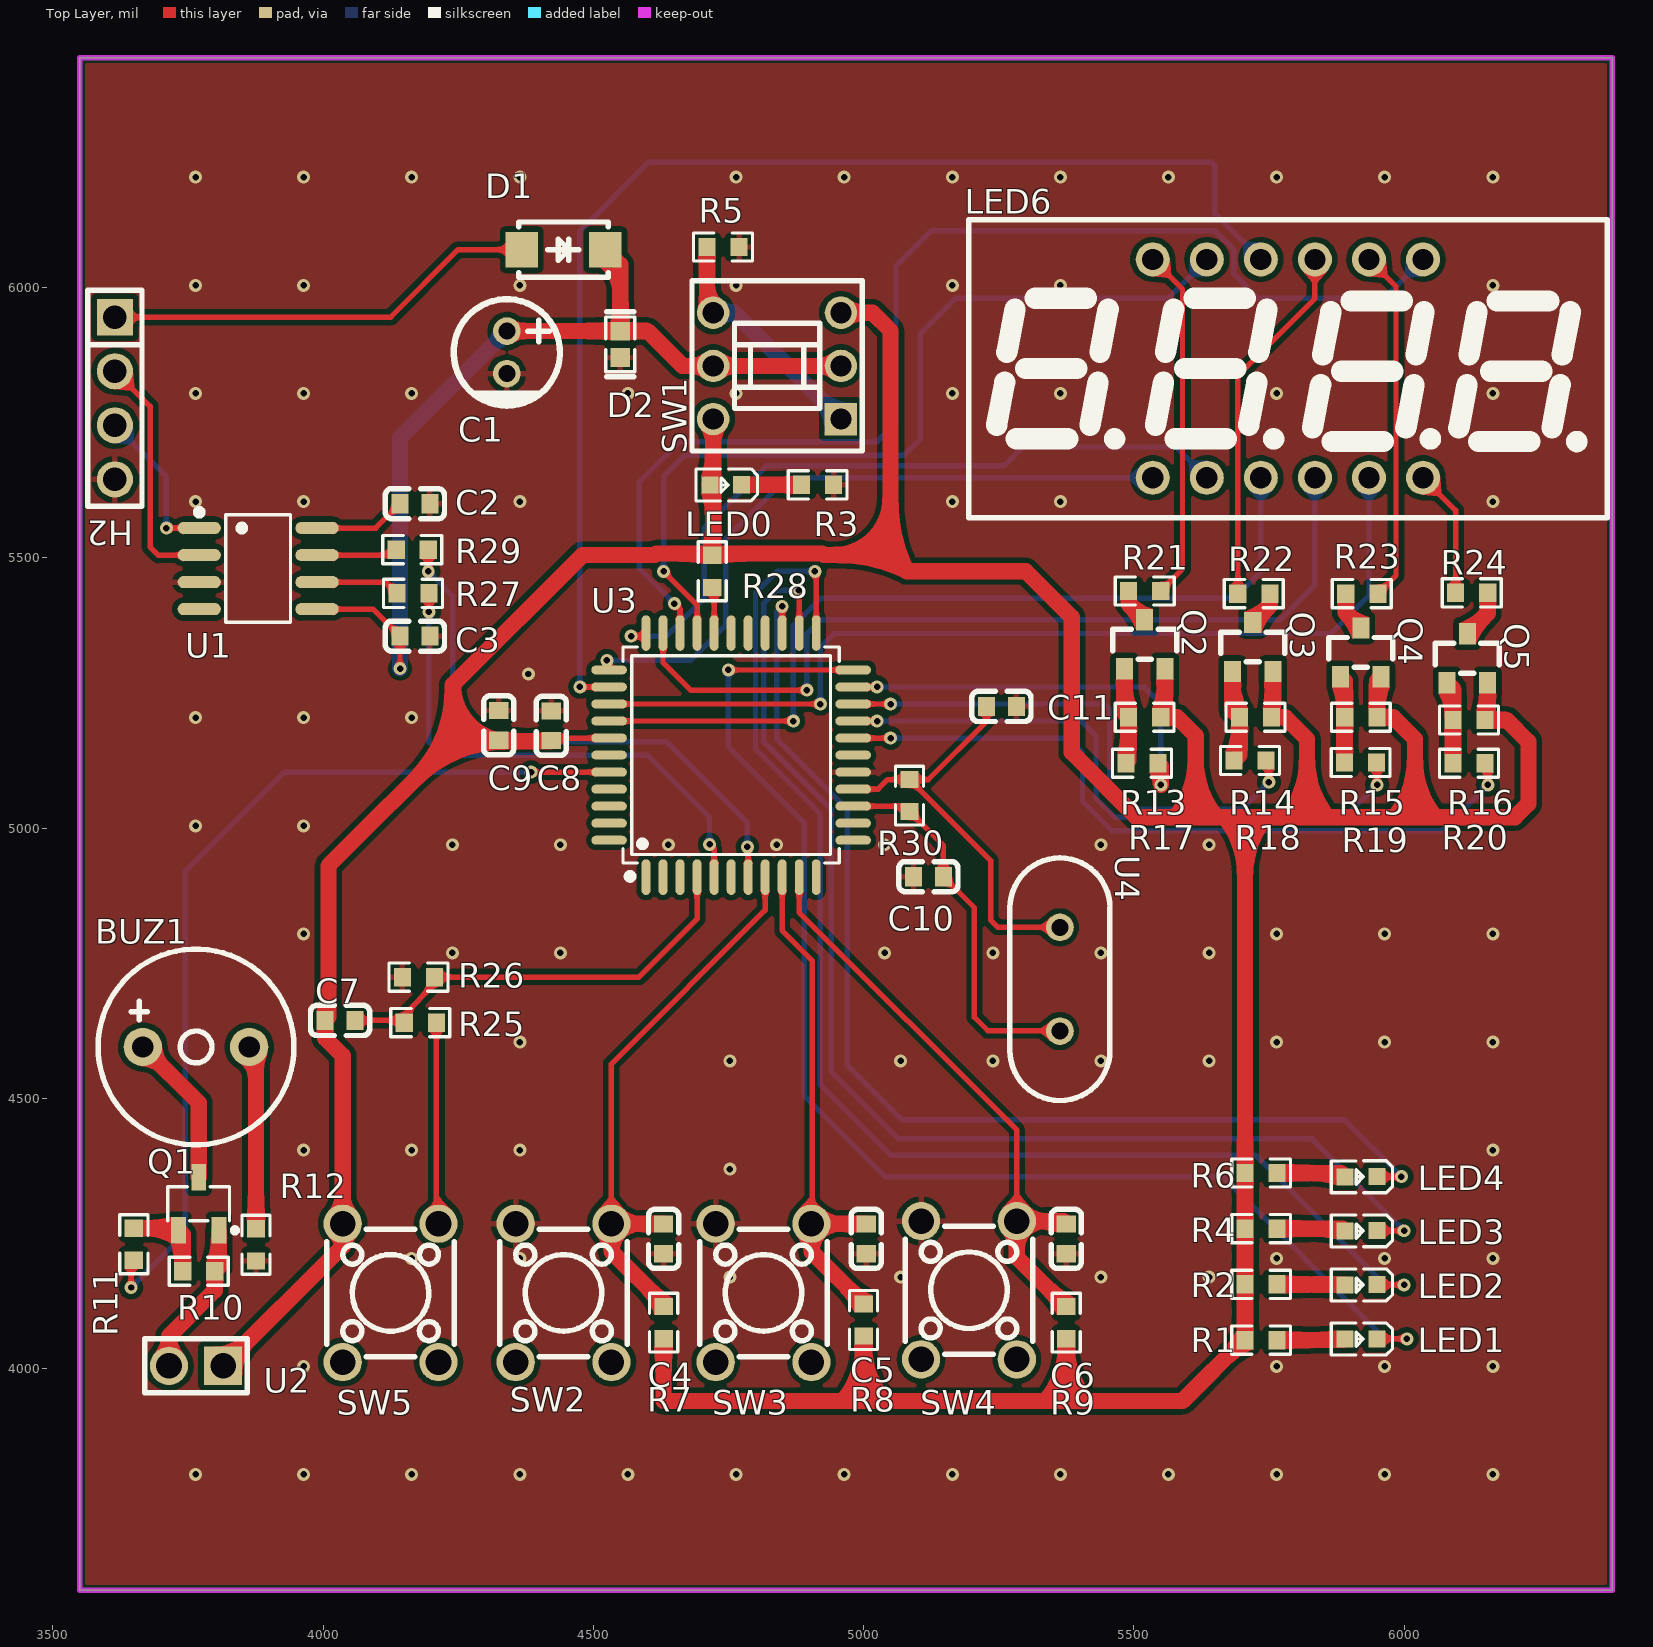
[diagram p0: Top Layer view]
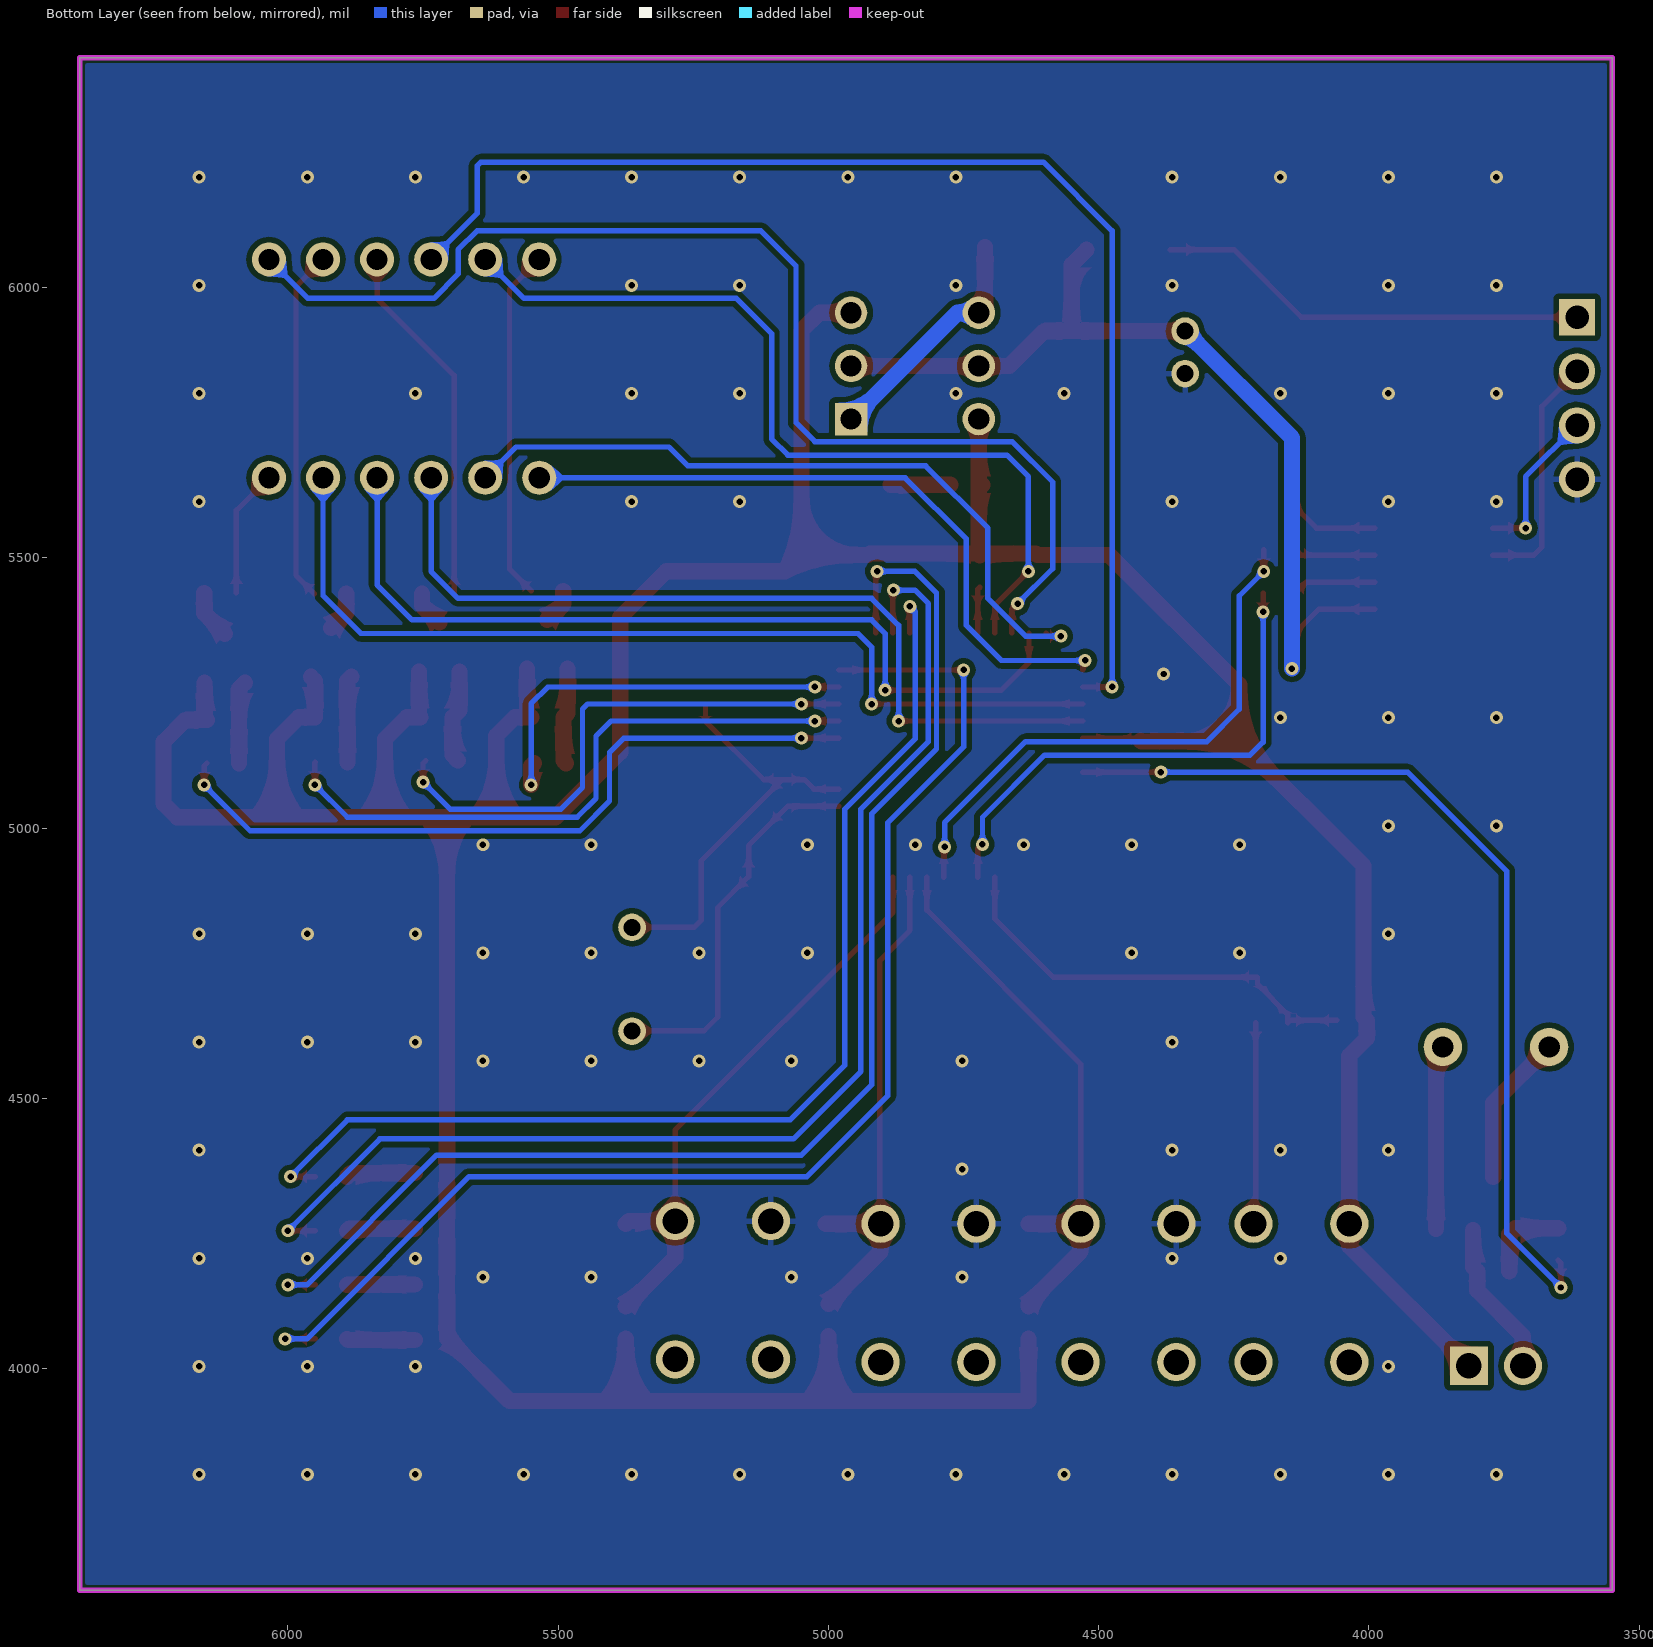
[diagram p1: Bottom Layer view, seen from below]
# Altium PCB MISC89012.pcbdoc
Units mil, origin at the board's own origin, x right, y up, seen from the top; angles counter-clockwise.
Board outline 2835 x 2835 mil, 2 copper layers (Top Layer, Bottom Layer), stack 62.206 mil thick; 65 components, 58 nets, 207 pads, 129 vias.

## Layer stack, top to bottom
Top Solder Mask Layer: solder mask 0.394, Dk 3.3
Top Layer: signal copper 1.379
Dielectric1: surface 59.449, FR4, Dk 4.5
Bottom Layer: signal copper 1.378
Bottom Solder Mask Layer: solder mask 0.394, Dk 3.3

## Board outline
3550,6425 3550,3590 6385,3590 6385,6425

## Design rules (kind name [scope] priority, off if disabled: settings)
BoardOutlineClearance copperThickness2oz_1 [All] p2 off: genericclearance=7.99 ignorepadtopadclearanceinfootprint=FALSE except(0: Arc-SplitContinuation Track-SplitContinuation SMDPad-SplitContinuation THPad-SplitContinuation Via-SplitContinuation Fill-SplitContinuation Region-SplitContinuation Poly-SplitContinuation Text-SplitContinuation Hole-SplitContinuation; 5.98: Arc-CutoutEdge SMDPad-CutoutEdge THPad-CutoutEdge Via-CutoutEdge Fill-CutoutEdge Region-CutoutEdge Text-CutoutEdge; 6.93: Hole-OutlineEdge Hole-CutoutEdge; 10: Poly-OutlineEdge Poly-CutoutEdge; 11.81: Arc-OutlineEdge Track-OutlineEdge SMDPad-OutlineEdge THPad-OutlineEdge Via-OutlineEdge Fill-OutlineEdge Region-OutlineEdge Text-OutlineEdge Track-CutoutEdge)
BoardOutlineClearance copperThickness1oz_1 [All] p4: genericclearance=4.02 ignorepadtopadclearanceinfootprint=FALSE except(0: Arc-SplitContinuation Track-SplitContinuation SMDPad-SplitContinuation THPad-SplitContinuation Via-SplitContinuation Fill-SplitContinuation Region-SplitContinuation Poly-SplitContinuation Text-SplitContinuation Hole-SplitContinuation; 6: SMDPad-CutoutEdge THPad-CutoutEdge Via-CutoutEdge Fill-CutoutEdge Region-CutoutEdge Text-CutoutEdge; 6.93: Hole-OutlineEdge Hole-CutoutEdge; 10: Poly-OutlineEdge Poly-CutoutEdge; 11.8: Arc-OutlineEdge Track-OutlineEdge SMDPad-OutlineEdge THPad-OutlineEdge Via-OutlineEdge Fill-OutlineEdge Region-OutlineEdge Text-OutlineEdge; 11.81: Arc-CutoutEdge Track-CutoutEdge)
Clearance copperThickness2oz [All] p1 off: gap=7.99 ignorepadtopadclearanceinfootprint=FALSE except(5.98: SMDPad-Track SMDPad-SMDPad THPad-Track SMDPad-THPad THPad-THPad Track-Via SMDPad-Via THPad-Via Via-Via Fill-Track Region-Track Fill-SMDPad Region-SMDPad Fill-THPad Region-THPad Fill-Via Region-Via Fill-Fill Fill-Region Region-Region Arc-Track Arc-SMDPad Arc-THPad Arc-Via Fill-Arc Region-Arc Arc-Arc Text-Track SMDPad-Text Text-THPad Text-Via Fill-Text Region-Text Arc-Text Text-Text; 6.93: Hole-Track Hole-SMDPad Hole-THPad Hole-Via Fill-Hole Region-Hole Hole-Arc Hole-Text; 10: Poly-Track Poly-SMDPad Poly-THPad Poly-Via Poly-Fill Poly-Region Poly-Poly Poly-Arc Poly-Text Poly-Hole)
Clearance copperThickness1oz [All] p3: gap=4.02 ignorepadtopadclearanceinfootprint=FALSE except(5.98: SMDPad-Track SMDPad-SMDPad THPad-Track SMDPad-THPad THPad-THPad Track-Via SMDPad-Via THPad-Via Via-Via Fill-Track Region-Track Fill-SMDPad Region-SMDPad Fill-THPad Region-THPad Fill-Via Region-Via Fill-Fill Fill-Region Region-Region; 6: Arc-Track Arc-SMDPad Arc-THPad Arc-Via Fill-Arc Region-Arc Arc-Arc Text-Track SMDPad-Text Text-THPad Text-Via Fill-Text Region-Text Arc-Text Text-Text; 6.93: Hole-Track Hole-SMDPad Hole-THPad Hole-Via Fill-Hole Region-Hole Hole-Arc Hole-Text; 10: Poly-Track Poly-SMDPad Poly-THPad Poly-Via Poly-Fill Poly-Region Poly-Poly Poly-Arc Poly-Text Poly-Hole)
Creepage creepage [All] p1: checkdistance=0 ignoreinternallayers=TRUE applytopolygonpour=TRUE
DiffPairsRouting differentialPair [All] p1: maxlimit=6 minlimit=6 mostfreqgap=6 toplayer_minwidth=5 toplayer_prefwidth=10 toplayer_maxwidth=100 toplayer_mingap=6 toplayer_prefgap=6 toplayer_maxgap=6 bottomlayer_minwidth=5 bottomlayer_prefwidth=10 bottomlayer_maxwidth=100 bottomlayer_mingap=6 bottomlayer_prefgap=6 bottomlayer_maxgap=6 maxuncoupledlength=10
HoleToHoleClearance otherClearance [All] p1: gap=11.81 allowstackedmicrovias=TRUE
Length netLength [All] p1: minlimit=0 maxlimit=0
MatchedLengths netLengthTolerance [All] p1: tolerance=1000
PasteMaskExpansion pasteMaskExpansion [All] p1: expansion=0
PlaneConnect innerPlane [All] p1: planeconnectstyle=Relief reliefexpansion=20 reliefentries=4 reliefconductorwidth=10 reliefairgap=10
PolygonConnect copperRegion [(InNet('GND'))] p1: connectstyle=Relief reliefconductorwidth=10 reliefentries=4 polygonreliefangle="90 Angle" airgapwidth=10 via.connectstyle=Relief via.reliefconductorwidth=10 via.reliefentries=4 via.polygonreliefangle="90 Angle" via.airgapwidth=10
RoutingVias viaSize [All] p1: holewidth=12.01 width=24.02 viastyle="Through Hole" minholewidth=11.81 minwidth=19.68 maxholewidth=248.03 maxwidth=393.7
SolderMaskExpansion solderMaskExpansion [IsVia] p1: expansion=-1000 istentingtop=TRUE
SolderMaskExpansion solderMaskExpansion [All] p2: expansion=2 istentingtop=FALSE
Width copperThickness2oz_2 [All] p1 off: maxlimit=100 minlimit=8 preferedwidth=10
Width copperThickness1oz_2 [All] p2: maxlimit=100 minlimit=5 preferedwidth=10

## Components (designator, comment, footprint, x,y, rotation, side; value= is the part's Value field where it differs from the comment)
BUZ1 "SUN-09055-3" BUZ-TH_BD9.0-P5.00-D0.6-FD 3765,4595 r0 top
C1 "100uF" CAP-TH_BD5.0-P2.00-D0.8-FD 4340,5880 r270 top
C2 "100nF" C0603 4170,5600 r0 top
C3 "100nF" C0603 4170,5355 r0 top
C4 "100nF" C0603 4630,4240 r90 top
C5 "100nF" C0603 5005,4240 r90 top
C6 "100nF" C0603 5375,4240 r90 top
C7 "10uF" C0603 4031.52,4644.16 r180 top
C8 "100nF" C0603 4422.16,5189.16 r270 top
C9 "10uF" C0603 4325,5190 r270 top
C10 "47pF" C0603 5120,4910 r0 top
C11 "47pF" C0603 5255,5225 r180 top
D1 "SS14" SMA_L4.2-W2.6-LS5.0-RD_1 4445,6070 r180 top
D2 "0603ESDA-05N" D0603-BI 4550,5895 r90 top
H2 "PZ254V-11-04P" HDR-TH_4P-P2.54-V-M 3615,5795 r270 top
LED0 "NCD0603R1" LED0603-RD_RED 4745,5635 r180 top
LED1 "NCD0603R1" LED0603-RD_RED 5920,4055 r180 top
LED2 "NCD0603R1" LED0603-RD_RED 5920,4155 r180 top
LED3 "NCD0603R1" LED0603-RD_RED 5920,4255 r180 top
LED4 "NCD0603R1" LED0603-RD_RED 5920,4355 r180 top
LED6 "SR410361N" LED-SEG-TH_12P-L30.0-W14.0-P2.54-S10.26-BL 5785,5850 r0 top
Q1 "2N3906S-RTK/P" SOT-23-3_L2.9-W1.6-P1.90-LS2.8-TR-CW 3770,4305 r270 top
Q2 "AO3401A" SOT-23_L2.9-W1.3-P1.90-LS2.4-BR 5520,5340 r270 top
Q3 "AO3401A" SOT-23_L2.9-W1.3-P1.90-LS2.4-BR 5720,5335 r270 top
Q4 "AO3401A" SOT-23_L2.9-W1.3-P1.90-LS2.4-BR 5920,5325 r270 top
Q5 "AO3401A" SOT-23_L2.9-W1.3-P1.90-LS2.4-BR 6116.97,5314.25 r270 top
R1 "4.7kΩ" R0603 5735.51,4052.65 r0 top
R2 "4.7kΩ" R0603 5735.51,4155.74 r0 top
R3 "4.7kΩ" R0603 4915,5635 r180 top
R4 "4.7kΩ" R0603 5735.51,4258.84 r0 top
R5 "2kΩ" R0603 4740,6075 r180 top
R6 "4.7kΩ" R0603 5735.51,4361.94 r0 top
R7 "10kΩ" R0603 4630,4085 r270 top
R8 "10kΩ" R0603 5000,4090 r270 top
R9 "10kΩ" R0603 5375,4085 r270 top
R10 "10kΩ" R0603 3770,4180 r0 top
R11 "1kΩ" R0603 3650,4230 r90 top
R12 "10Ω" R0603 3876.06,4228.97 r90 top
R13 "10kΩ" R0603 5520,5205 r0 top
R14 "10kΩ" R0603 5725,5205 r0 top
R15 "10kΩ" R0603 5920,5205 r0 top
R16 "10kΩ" R0603 6120,5200 r0 top
R17 "1kΩ" R0603 5515,5120 r180 top
R18 "1kΩ" R0603 5715,5125 r180 top
R19 "1kΩ" R0603 5919.55,5121.38 r0 top
R20 "1kΩ" R0603 6120,5120 r0 top
R21 "47Ω" R0603 5520.1,5438.62 r180 top
R22 "47Ω" R0603 5722.02,5433.62 r0 top
R23 "47Ω" R0603 5921.77,5433.62 r180 top
R24 "47Ω" R0603 6125,5435 r0 top
R25 "100Ω" R0603 4180,4640 r0 top
R26 "10kΩ" R0603 4176.52,4724.16 r0 top
R27 "1kΩ" R0603 4166.27,5434.16 r0 top
R28 "10kΩ" R0603 4720,5475 r90 top
R29 "1kΩ" R0603 4165,5515 r0 top
R30 "1MΩ" R0603 5085,5060 r270 top
SW1 "XKB8080-Z" SW-TH_6P-L8.0-W8.0-P2.50 4840,5855 r90 top
SW2 "TS-1095-A5B2-D1" SW-TH_4P-L6.0-W6.0-P4.50-LS6.5 4445,4140 r270 top
SW3 "TS-1095-A5B2-D1" SW-TH_4P-L6.0-W6.0-P4.50-LS6.5 4815,4140 r270 top
SW4 "TS-1095-A5B2-D1" SW-TH_4P-L6.0-W6.0-P4.50-LS6.5 5195,4145 r270 top
SW5 "TS-1095-A5B2-D1" SW-TH_4P-L6.0-W6.0-P4.50-LS6.5 4125,4140 r90 top
U1 "CH340N" SOP-8_L5.0-W4.0-P1.27-LS6.0-BL 3880,5480 r270 top
U2 "54102-T0600LF" HDR-TH_2P-P2.54-V-M-R2-C1-S2.54 3765,4005 r90 top
U3 "STC89C52RC-40I-LQFP44" LQFP-44_L10.0-W10.0-P0.80-LS12.0-BL 4755,5135 r0 top
U4 "12MHz" HC-49S_L11.4-W4.7-P4.88-D0.4 5363.3,4720.32 r270 top

## Footprints (in the part's own frame and the unit in brackets; to place one, negate y for a bottom-side part, rotate by r counter-clockwise, add the part's x,y. Pads: shape width x height; smd on the part's side, far side on the other; paste and mask are expansions set on the pad)
BUZ-TH_BD9.0-P5.00-D0.6-FD [mm]
  round 1.8 hole 1 copper offset 0,0: 1(-2.5,0)
  round 1.8 hole 1: 2(2.5,0)
  silkscreen extent -4.6,-4.6 4.6,4.6
C0603 [mm]
  rect 0.8x0.9 smd: 1(-0.7,0) 2(0.7,0)
  silkscreen extent -1.39,-0.71 1.39,0.71
CAP-TH_BD5.0-P2.00-D0.8-FD [mm]
  round 1.3 hole 0.8: 1(-1,0) 2(1,0)
  silkscreen extent -2.5,-2.5 2.5,2.5
D0603-BI [mil]
  rect 34.38x35.72 smd paste-3937.01 mask+2: 1(-24.47,0) 2(24.47,0)
  silkscreen extent -60,-27 60,27
HC-49S_L11.4-W4.7-P4.88-D0.4 [mm]
  round 1.3 hole 0.8 paste+0 mask+0.05: 1(-2.44,0) 2(2.44,0)
  silkscreen extent -5.7,-2.35 5.7,2.35
HDR-TH_2P-P2.54-V-M-R2-C1-S2.54 [mm]
  rect 1.8x1.8 hole 1.2: 1(0,-1.27)
  round 1.8 hole 1.2: 2(0,1.27)
  silkscreen extent -1.27,-2.41 1.27,2.41
HDR-TH_4P-P2.54-V-M [mm]
  rect 1.7x1.7 hole 1.1: 1(-3.81,0)
  round 1.7 hole 1.1: 2(-1.27,0) 3(1.27,0) 4(3.81,0)
  silkscreen extent -5.08,-1.27 5.08,1.27
LED0603-RD_RED [mm]
  rect 0.8x0.8 smd: 1(-0.749,-0.003) 2(0.749,0.003)
  silkscreen extent -1.49,-0.75 1.39,0.76
LED-SEG-TH_12P-L30.0-W14.0-P2.54-S10.26-BL [mm]
  round 1.6 hole 1: 1(-6.35,-5.13) 2(-3.81,-5.13) 3(-1.27,-5.13) 4(1.27,-5.13) 5(3.81,-5.13) 6(6.35,-5.13) 7(6.35,5.13) 8(3.81,5.13) 9(1.27,5.13) 10(-1.27,5.13) 11(-3.81,5.13) 12(-6.35,5.13)
  silkscreen extent -15,-7 15,7
LQFP-44_L10.0-W10.0-P0.80-LS12.0-BL [mm]
  oval 0.42x1.67 smd: 1(-4,-5.735) 2(-3.2,-5.735) 3(-2.4,-5.735) 4(-1.6,-5.735) 5(-0.8,-5.735) 6(0,-5.735) 7(0.8,-5.735) 8(1.6,-5.735) 9(2.4,-5.735) 10(3.2,-5.735) 11(4,-5.735) 23(4,5.735) 24(3.2,5.735) 25(2.4,5.735) 26(1.6,5.735) 27(0.8,5.735) 28(0,5.735) 29(-0.8,5.735) 30(-1.6,5.735) 31(-2.4,5.735) 32(-3.2,5.735) 33(-4,5.735)
  oval 1.67x0.42 smd: 12(5.735,-4) 13(5.735,-3.2) 14(5.735,-2.4) 15(5.735,-1.6) 16(5.735,-0.8) 17(5.735,0) 18(5.735,0.8) 19(5.735,1.6) 20(5.735,2.4) 21(5.735,3.2) 22(5.735,4) 34(-5.735,4) 35(-5.735,3.2) 36(-5.735,2.4) 37(-5.735,1.6) 38(-5.735,0.8) 39(-5.735,0) 40(-5.735,-0.8) 41(-5.735,-1.6) 42(-5.735,-2.4) 43(-5.735,-3.2) 44(-5.735,-4)
  silkscreen extent -5.08,-5.85 5.08,5.08
R0603 [mil]
  rect 31.75x34.02 smd paste-3937.01 mask+2: 1(-29.66,0) 2(29.66,0)
  silkscreen extent -55,-26 55,26
SMA_L4.2-W2.6-LS5.0-RD_1 [mm]
  rect 1.52x1.68 smd: 1(-1.965,0) 2(1.965,0)
  silkscreen extent -2.1,-1.3 2.1,1.3
SOP-8_L5.0-W4.0-P1.27-LS6.0-BL [mil]
  oval 22.6x80.14 smd: 1(-75,-108.97) 2(-25,-108.97) 3(25,-108.97) 4(75,-108.97) 5(75,108.97) 6(25,108.97) 7(-25,108.97) 8(-75,108.97)
  silkscreen extent -110,-115 99,60
SOT-23-3_L2.9-W1.6-P1.90-LS2.8-TR-CW [mm]
  rect 1.25x0.7 smd: 1(1.25,0.95) 2(1.25,-0.95) 3(-1.25,0)
  silkscreen extent -0.8,-1.45 1.37,1.82
SOT-23_L2.9-W1.3-P1.90-LS2.4-BR [mm]
  rect 1x0.8 smd: 1(1.15,-0.95) 2(1.15,0.95) 3(-1.15,0)
  silkscreen extent -0.7,-1.5 0.7,1.5
SW-TH_4P-L6.0-W6.0-P4.50-LS6.5 [mm]
  round 1.8 hole 1.2: 1(-3.25,2.25) 2(3.25,2.25) 3(-3.25,-2.25) 4(3.25,-2.25)
  silkscreen extent -3,-3 3,3
SW-TH_6P-L8.0-W8.0-P2.50 [mm]
  rect 1.524x1.524 hole 1: 1(-2.5,-3)
  round 1.524 hole 1: 2(0,-3) 3(2.5,-3) 4(-2.5,3) 5(0,3) 6(2.5,3)
  silkscreen extent -4,-4 4,4

## Via types
v1: diameter 24.02, hole 12, Top Layer to Bottom Layer, 129 vias

## Nets (pads, with @x,y where several pads share a name; then routed paths per layer and width w, separated by ;. In a path a pad name is that pad's centre, name@x,y a point inside that pad or via, vN(x,y) a via of type N, cw(c..) or ccw(c..) an arc to the next point about the centre after c; other vN are vias at no path point)
$1N1: D1.2 H2.1 | length 804.4
  Top Layer w10: H2.1 4125,5945 4250,6070 D1.2
$1N12: C2.1 U1.8 | length 172.1
  Top Layer w10: U1.8 4097.44,5555 C2.1
$1N15: LED0.1 R3.2 | length 110.9
  Top Layer w30: LED0.1 4885.2,5635.14 R3.2
$1N23: R5.2 SW1.1 SW1.6 | length 444.1
  Top Layer w30: R5.2 4710.34,5964.98 SW1.6
  Bottom Layer w30: SW1.6 4761.26,5953.43 SW1.1
$1N27: LED1.2 R1.2 | length 126.3
  Top Layer w30: R1.2 5888.29,4052.65 LED1.2
$1N28: LED2.2 R2.2 | length 125.7
  Top Layer w30: R2.2 5889.63,4155.74 LED2.2
$1N29: LED3.2 R4.2 | length 127
  Top Layer w30: R4.2 5886.54,4258.84 LED3.2
$1N30: LED4.2 R6.2 | length 128.3
  Top Layer w30: R6.2 5883.44,4361.94 LED4.2
$1N45: BUZ1.2 R12.2 | length 341.6
  Top Layer w30: BUZ1.2 3876.06,4582.36 R12.2
$1N47: BUZ1.1 Q1.3 | length 283.6
  Top Layer w30: BUZ1.1 3770,4491.57 Q1.3
$1N48: Q1.2 R10.1 R11.2 | length 163.2
  Top Layer w30: R11.2 3728.74,4259.66 Q1.2 3740.34,4248.06 R10.1
$1N50: Q1.1 R10.2 U2.2 | length 289.1
  Top Layer w30: U2.2 3715,4060 3799.66,4144.66 R10.2 3807.4,4187.74 Q1.1
$1N61: R28.1 U3.29 | length 86
  Top Layer w10: R28.1 4723.5,5441.84 U3.29
$1N75: R27.2 U3.5 | length 966.1
  Top Layer w10: v1(4195.93,5400) R27.2 ; v1(4715,4970) 4723.5,4961.5 U3.5
  Bottom Layer w10: v1(4195.93,5400) 4195.93,5159.07 4220,5135 4600,5135 4715,5020 v1(4715,4970)
$1N76: R29.2 U3.7 | length 1047.2
  Top Layer w10: v1(4194.66,5475) R29.2 ; v1(4785,4965) 4786.5,4963.5 U3.7
  Bottom Layer w10: v1(4194.66,5475) 4240,5429.66 4240,5220 4300,5160 4635,5160 4785,5010 v1(4785,4965)
$1N86: R25.2 SW5.4 | length 373.7
  Top Layer w10: R25.2 4209.66,4271.87 SW5.4
$1N99: Q2.1 R13.1 R17.2 | length 180
  Top Layer w30: Q2.1 5482.6,5212.74 R13.1 5490.34,5125 R17.2
$1N101: Q3.1 R14.1 R18.2 | length 174.1
  Top Layer w30: Q3.1 5682.6,5217.74 R14.1 5695.34,5135 R18.2
$1N104: Q5.1 R16.1 R20.1 | length 153.4
  Top Layer w30: Q5.1 6090.34,5258.21 R16.1 R20.1
$1N106: Q4.1 R15.1 R19.1 | length 161.7
  Top Layer w30: Q4.1 5890.34,5271.98 R15.1 5889.89,5204.55 R19.1
$1N115: LED6.12 R21.1 | length 652.8
  Top Layer w10: LED6.12 5590,5996.97 5590,5478.87 R21.1
$1N116: LED6.9 R22.1 | length 677.4
  Top Layer w10: R22.1 5692.36,5837.36 5835,5980 LED6.9
$1N117: LED6.8 R23.1 | length 653
  Top Layer w10: LED6.8 5985,6001.97 5985,5467.2 R23.1
$1N118: LED6.6 R24.1 | length 238
  Top Layer w10: LED6.6 6095.34,5587.69 R24.1
$1N120: C10.2 R30.2 U3.14 U4.2 | length 707.4
  Top Layer w10: U3.14 5074.83,5040.51 R30.2 5147.56,4967.78 C10.2 5205,4852.56 5205,4650 5230,4625 5362.56,4625 U4.2
$1N121: C11.2 R30.1 U3.15 U4.1 | length 781.9
  Top Layer w10: U3.15 5027.01,5072.01 5044.66,5089.66 R30.1 ; C11.2 5227.44,5197.44 5119.66,5089.66 R30.1 ; U4.1 5248.62,4816.38 5235,4830 5235,4939.66 R30.1
$1N123: Q2.3 R21.2 | length 65.6
  Top Layer w30: R21.2 5490.44,5414.84 Q2.3
$1N124: Q3.3 R22.2 | length 66.5
  Top Layer w30: Q3.3 5751.68,5411.95 R22.2
$1N125: Q4.3 R23.2 | length 74.9
  Top Layer w30: R23.2 5892.11,5398.17 Q4.3
$1N126: Q5.3 R24.2 | length 91.1
  Top Layer w30: Q5.3 6154.66,5397.21 R24.2
BEEP: R11.1 U3.40 | length 1724.1
  Top Layer w10: v1(3645,4150) 3645,4195.34 R11.1 ; v1(4385,5103.5) U3.40
  Bottom Layer w10: v1(3645,4150) 3745,4250 3745,4920 3928.5,5103.5 v1(4385,5103.5)
D+: H2.3 U1.1 | length 290.4
  Top Layer w10: v1(3710,5555) U1.1
  Bottom Layer w10: H2.3 3710,5650 v1(3710,5555)
D-: H2.2 U1.2 | length 449.2
  Top Layer w10: H2.2 3680,5780 3680,5520 3695,5505 U1.2
GND: C1.2 C2.2 C3.2 C4.1 C5.1 C6.1 C8.1 C9.1 C10.1 C11.1 D2.1 H2.4 R3.1 R5.1 R12.1 R26.1 SW2.3 SW3.3 SW4.3 U1.3 U3.16
  other v1: 3764.1,3804.1 3964.1,3804.1 4164.1,3804.1 4364.1,3804.1 4564.1,3804.1 4764.1,3804.1 4964.1,3804.1 5164.1,3804.1 5364.1,3804.1 5564.1,3804.1 5764.1,3804.1 5964.1,3804.1 6164.1,3804.1 3964.1,4004.1 5764.1,4004.1 5964.1,4004.1 6164.1,4004.1 4752.68,4169.1 5068.59,4169.1 5439.1,4169.1 5639.1,4169.1 4164.1,4204.1 4364.1,4204.1 5764.1,4204.1 5964.1,4204.1 6164.1,4204.1 4752.68,4369.1 3964.1,4404.1 4164.1,4404.1 4364.1,4404.1 6164.1,4404.1 4752.68,4569.1 5068.59,4569.1 5239.1,4569.1 5439.1,4569.1 5639.1,4569.1 4364.1,4604.1 5764.1,4604.1 5964.1,4604.1 6164.1,4604.1 4239.1,4769.1 4439.1,4769.1 5039.1,4769.1 5239.1,4769.1 5439.1,4769.1 5639.1,4769.1 3964.1,4804.1 5764.1,4804.1 5964.1,4804.1 6164.1,4804.1 4239.1,4969.1 4439.1,4969.1 4639.1,4969.1 4839.1,4969.1 5039.1,4969.1 5439.1,4969.1 5639.1,4969.1 3764.1,5004.1 3964.1,5004.1 3764.1,5204.1 3964.1,5204.1 4164.1,5204.1 4380,5285 3764.1,5604.1 3964.1,5604.1 4364.1,5604.1 5164.1,5604.1 5364.1,5604.1 6164.1,5604.1 3764.1,5804.1 3964.1,5804.1 4164.1,5804.1 4564.1,5804.1 4764.1,5804.1 5164.1,5804.1 5364.1,5804.1 5764.1,5804.1 6164.1,5804.1 3764.1,6004.1 3964.1,6004.1 4364.1,6004.1 4764.1,6004.1 5164.1,6004.1 5364.1,6004.1 6164.1,6004.1 3764.1,6204.1 3964.1,6204.1 4164.1,6204.1 4364.1,6204.1 4764.1,6204.1 4964.1,6204.1 5164.1,6204.1 5364.1,6204.1 5564.1,6204.1 5764.1,6204.1 5964.1,6204.1 6164.1,6204.1
KEY1: C4.2 R7.1 SW2.1 U3.8 | length 1048.9
  Top Layer w10: SW2.1 4533.58,4563.58 4817.99,4847.99 U3.8
  Top Layer w30: R7.1 4630,4120 4533.58,4216.42 SW2.1 4629.61,4267.95 C4.2
KEY2: C5.2 R8.1 SW3.1 U3.9 | length 954.7
  Top Layer w10: U3.9 4849.49,4810.51 4905,4755 4905,4269.37 SW3.1
  Top Layer w30: R8.1 4903.58,4216.08 SW3.1 5004.61,4267.95 C5.2
KEY3: C6.2 R9.1 SW4.1 U3.10 | length 1092.8
  Top Layer w10: U3.10 4880.98,4844.02 5283.58,4441.42 SW4.1
  Top Layer w30: R9.1 5283.58,4206.08 SW4.1 5369.61,4272.95 C6.2
LED1: LED1.1 U3.22 | length 2433.2
  Top Layer w10: v1(4750,5292.48) U3.22 ; LED1.1 5949.62,4055 v1(6005,4055)
  Bottom Layer w10: v1(4750,5292.48) 4750,5150 4890,5010 4890,4505 5040,4355 5665,4355 5965,4055 v1(6005,4055)
LED2: LED2.1 U3.23 | length 2485.3
  Top Layer w10: v1(4910,5475) 4912.48,5472.52 U3.23 ; LED2.1 5949.62,4155 v1(6000,4155)
  Bottom Layer w10: v1(4910,5475) 4840,5475 4800,5435 4800,5146.42 4920,5026.42 4920,4525 5050,4395 5725,4395 5965,4155 v1(6000,4155)
LED3: LED3.1 U3.24 | length 2304.5
  Top Layer w10: v1(4880,5440) 4880.98,5439.02 U3.24 ; LED3.1 5949.62,4255 v1(6000,4255)
  Bottom Layer w10: v1(4880,5440) 4840,5440 4815,5415 4815,5160 4940,5035 4940,4550 5065,4425 5830,4425 v1(6000,4255)
LED4: LED4.1 U3.25 | length 2112.4
  Top Layer w10: U3.25 v1(4849.49,5410) ; LED4.1 5949.62,4355 v1(5995,4355)
  Bottom Layer w10: v1(4849.49,5410) 4839.49,5400 4839.49,5165 4970,5034.49 4970,4560.77 5070.77,4460 5890,4460 v1(5995,4355)
NETB: LED6.7 U3.31 | length 2230.9
  Top Layer w10: v1(4650,5415) 4660.51,5404.49 U3.31
  Bottom Layer w10: v1(4650,5415) 4585,5480 4585,5640 4660,5715 5025,5715 5060,5750 5060,6040 5125,6105 5650,6105 5685,6070 5685,6025 5730,5980 5963.03,5980 LED6.7
NETC: LED6.4 U3.32 | length 1622.2
  Top Layer w10: U3.32 4629.02,5305.98 4680,5255 v1(4895,5255)
  Bottom Layer w10: v1(4895,5255) 4895,5360 4920,5385 5770,5385 5835,5450 LED6.4
NETD: LED6.2 U3.33 | length 1339.6
  Top Layer w10: v1(4570,5355) 4591.73,5355 U3.33
  Bottom Layer w10: v1(4570,5355) 4635,5355 4705,5425 4705,5555 4820,5670 5260,5670 5295,5705 5578.03,5705 LED6.2
NETDP: LED6.3 U3.37 | length 1597.3
  Top Layer w10: U3.37 v1(4870,5197.99)
  Bottom Layer w10: v1(4870,5197.99) 4870,5375 4920,5425 5685,5425 5735,5475 LED6.3
NETE: LED6.1 U3.34 | length 1263
  Top Layer w10: v1(4525,5310) 4529.21,5305.79 U3.34
  Bottom Layer w10: v1(4525,5310) 4680,5310 4745,5375 4745,5535 4858.03,5648.03 LED6.1
NETF: LED6.10 U3.35 | length 2337
  Top Layer w10: v1(4475,5260.98) U3.35
  Bottom Layer w10: v1(4475,5260.98) 4475,6105 4602.07,6232.07 5642.93,6232.07 5650,6225 5650,6136.97 LED6.10
NETG: LED6.5 U3.36 | length 1768.7
  Top Layer w10: U3.36 v1(4920,5229.49)
  Bottom Layer w10: v1(4920,5229.49) 4920,5335 4945,5360 5865,5360 5935,5430 LED6.5
RST: C7.1 R25.1 R26.2 U3.4 | length 808
  Top Layer w10: C7.1 4146.18,4644.16 R25.1 4150.34,4655.34 4206.18,4711.18 R26.2 4584.16,4724.16 4692.01,4832.01 U3.4
RXD: R27.1 U1.6 | length 156.3
  Top Layer w10: U1.6 4115.76,5455 R27.1
SEGA: LED6.11 U3.30 | length 1600.6
  Top Layer w10: v1(4630,5475) 4692.01,5412.99 U3.30
  Bottom Layer w10: v1(4630,5475) 4630,5650 4670,5690 5075,5690 5105,5720 5105,5915 5170,5980 5563.03,5980 LED6.11
SEL0: R20.2 U3.18 | length 1375.4
  Top Layer w10: U3.18 v1(5050,5166.5) ; R20.2 6155,5114.66 v1(6155,5080)
  Bottom Layer w10: v1(5050,5166.5) 5378.5,5166.5 5405,5140 5405,5050 5460,4995 6070,4995 v1(6155,5080)
SEL1: R19.2 U3.19 | length 1176.9
  Top Layer w10: U3.19 v1(5025,5197.99) ; R19.2 5950,5120.58 v1(5950,5080)
  Bottom Layer w10: v1(5025,5197.99) 5402.01,5197.99 5430,5170 5430,5055 5465,5020 5890,5020 v1(5950,5080)
SEL2: R18.1 U3.20 | length 997.6
  Top Layer w10: U3.20 v1(5050,5229.49) ; R18.1 5750,5119.66 v1(5750,5085)
  Bottom Layer w10: v1(5050,5229.49) 5445.51,5229.49 5455,5220 5455,5075 5495,5035 5700,5035 v1(5750,5085)
SEL3: R17.1 U3.21 | length 774.3
  Top Layer w10: U3.21 v1(5025,5260.98)
  Top Layer w30: R17.1 5550,5114.66 v1(5550,5080)
  Bottom Layer w10: v1(5025,5260.98) 5519.02,5260.98 5550,5230 v1(5550,5080)
TXD: R29.1 U1.7 | length 150.5
  Top Layer w10: U1.7 4125.34,5505 R29.1
USB_IN: C1.1 C3.1 D1.1 D2.2 SW1.2 SW1.5 U1.5 | length 1747.2
  Top Layer w10: U1.5 4092.44,5405 C3.1 v1(4142.44,5295)
  Top Layer w30: C1.1 4549.9,5919.37 D2.2 ; D1.1 4550,6042.36 D2.2 ; SW1.2 SW1.5 4664.99,5855.01 4600.53,5919.47 D2.2
  Bottom Layer w30: v1(4142.44,5295) 4142.44,5721.81 C1.1
VCC: C7.2 C8.2 C9.2 LED0.2 Q2.2 Q3.2 Q4.2 Q5.2 R1.1 R2.1 R4.1 R6.1 R7.2 R8.2 R9.2 R13.2 R14.2 R15.2 R16.2 R28.2 SW1.3 SW1.4 SW5.2 U2.1 U3.38 | length 8648.5
  Top Layer w10: C8.2@4427.06,5166.5 U3.38
  Top Layer w30: U2.1 4036.42,4226.42 SW5.2 4036.42,4578.58 4003.96,4611.04 C7.2 4010,4650.2 4010,4930 4240,5160 ; C8.2 4420.56,5160 4240,5160 ; R7.2 4630,3940 4999.91,3940 ; LED0.2 LED0.2@4721.89,5641.24 ; R28.2 4721.89,5506.55 R28.2@4721.89,5507.99 ; SW1.4 LED0.2@4721.89,5641.24 ; SW1.3 5016.57,5953.43 5050,5920 5050,5505 ; R8.2 5000,3940.09 4999.91,3940 ; R9.2 5375,3940 ; Q2.2 5557.4,5212.74 R13.2 5580,5205 5614.42,5170.58 5614.42,5020 ; Q3.2 5757.4,5207.74 R14.2 5780,5205 5820.5,5164.5 5820.5,5020 ; Q4.2 5949.66,5271.98 R15.2 5980,5205 6020,5165 6020,5022.64 6022.64,5020 ; Q5.2 6154.37,5204.71 R16.2 6190,5200 6230,5160 6230,5045 6205,5020 6022.64,5020 ; 4240,5160 4240,5265 4480,5505 4613.34,5505 4616.33,5507.99 R28.2@4721.89,5507.99 ; R28.2@4721.89,5507.99 LED0.2@4721.89,5641.24 ; R28.2@4721.89,5507.99 4923.67,5507.99 4926.66,5505 5050,5505 ; 4999.91,3940 5375,3940 ; 5050,5505 5080,5475 5300,5475 5385,5390 5385,5140 5505,5020 5614.42,5020 ; 5375,3940 5590,3940 5705.85,4055.85 R2.1 R4.1 R6.1 5705.85,5019.34 5705.18,5020 ; 5614.42,5020 5705.18,5020 ; 5705.18,5020 5820.5,5020 ; 5820.5,5020 6022.64,5020
pads on no net: SW2.2 SW2.4 SW3.2 SW3.4 SW4.2 SW4.4 SW5.1 SW5.3 U1.4 U3.1 U3.2 U3.3 U3.6 U3.11 U3.12 U3.13 U3.17 U3.26 U3.27 U3.28 U3.39 U3.41 U3.42 U3.43 U3.44

## Polygon pours and split planes (outlines as drawn)
GND on Bottom Layer (solid, remove dead copper, pour order 2): 3000,6940 3000,3000 7020,3000 7020,6940
GND on Top Layer (solid, remove dead copper, pour order 0): 3250,6735 3250,3285 6870,3285 6870,6735

## Keep-outs
Board Outline Layer:
  the board outline again, w10

## Other copper
Top Layer:
  drawing of 222 lines, arcs and shapes, not listed
Bottom Layer:
  region net USB_IN: 4325.97,5884.13 4304.76,5905.34 4306.5,5907.22 4308.21,5909.3 4311.28,5913.72 4312.53,5915.86 4313.51,5917.85 4314.18,5919.58 4314.46,5920.97 4341.6,5893.83 4340.21,5893.55 4338.48,5892.88 4336.49,5891.9 4334.35,5890.65 4329.93,5887.58 4327.85,5885.87
  region net D+: 3650.75,5716.32 3643.68,5709.25 3640.91,5709.58 3633.89,5710.15 3612.9,5711.6 3648.4,5747.1 3649.85,5726.11 3650.42,5719.09
  region net SEGA: 5608.21,6018.11 5601.14,6025.18 5601.54,6027.84 5602.15,6034.42 5603.57,6053.94 5636.97,6020.54 5617.45,6019.12 5610.87,6018.51
  region net NETF: 5701.14,6078.76 5708.21,6085.83 5710.87,6085.43 5717.45,6084.82 5736.97,6083.4 5703.57,6050 5702.15,6069.52 5701.54,6076.1
  region net NETB: 6008.21,6018.11 6001.14,6025.18 6001.54,6027.84 6002.15,6034.42 6003.57,6053.94 6036.97,6020.54 6017.45,6019.12 6010.87,6018.51
  region net NETG: 5940,5605.15 5930,5605.15 5928.4,5607.31 5924.18,5612.39 5911.38,5627.2 5958.62,5627.2 5945.82,5612.39 5941.6,5607.31
  region net NETC: 5840,5605.15 5830,5605.15 5828.4,5607.31 5824.18,5612.39 5811.38,5627.2 5858.62,5627.2 5845.82,5612.39 5841.6,5607.31
  region net NETDP: 5740,5605.15 5730,5605.15 5728.4,5607.31 5724.18,5612.39 5711.38,5627.2 5758.62,5627.2 5745.82,5612.39 5741.6,5607.31
  region net NETD: 5601.14,5674.82 5608.21,5681.89 5610.87,5681.49 5617.45,5680.88 5636.97,5679.46 5603.57,5646.06 5602.15,5665.58 5601.54,5672.16
  region net NETE: 5492.12,5643.03 5492.12,5653.03 5494.28,5654.63 5499.36,5658.85 5514.17,5671.65 5514.17,5624.41 5499.36,5637.21 5494.28,5641.43
  region net $1N23: 4912.2,5781.27 4933.41,5802.48 4939.46,5798.37 4945.85,5794.83 4952.55,5791.89 4959.48,5789.58 4966.6,5787.92 4973.84,5786.91 4981.14,5786.57 4928.11,5733.54 4927.77,5740.84 4926.77,5748.09 4925.1,5755.2 4922.79,5762.14 4919.85,5768.83 4916.31,5775.23 4912.2,5781.27
  region net $1N23: 4761.26,5968.43 4761.26,5938.43 4759.01,5938.26 4756.48,5937.78 4753.78,5937.04 4751.02,5936.08 4748.33,5934.95 4745.8,5933.68 4743.57,5932.32 4741.73,5930.93 4741.73,5975.93 4743.57,5974.53 4745.8,5973.17 4748.33,5971.9 4751.02,5970.77 4753.78,5969.81 4756.48,5969.07 4759.01,5968.59
  region net SEGA: 4625,5491.35 4635,5491.35 4635.34,5489.54 4636.25,5487.27 4637.53,5484.94 4639.01,5482.94 4620.99,5482.94 4622.47,5484.94 4623.75,5487.27 4624.66,5489.54
  region net NETB: 4634.9,5423.02 4641.98,5430.1 4643.5,5429.06 4645.74,5428.1 4648.3,5427.36 4650.75,5426.98 4638.02,5414.25 4637.64,5416.7 4636.9,5419.26 4635.94,5421.5
  region net NETD: 4586.35,5360 4586.35,5350 4584.54,5349.66 4582.27,5348.75 4579.94,5347.47 4577.94,5345.99 4577.94,5364.01 4579.94,5362.53 4582.27,5361.25 4584.54,5360.34
  region net NETE: 4541.35,5315 4541.35,5305 4539.54,5304.66 4537.27,5303.75 4534.94,5302.47 4532.94,5300.99 4532.94,5319.01 4534.94,5317.53 4537.27,5316.25 4539.54,5315.34
  region net NETF: 4470,5277.33 4480,5277.33 4480.34,5275.52 4481.25,5273.25 4482.53,5270.92 4484.01,5268.92 4465.99,5268.92 4467.47,5270.92 4468.75,5273.25 4469.66,5275.52
  region net NETC: 4890,5271.35 4900,5271.35 4900.34,5269.54 4901.25,5267.27 4902.53,5264.94 4904.01,5262.94 4885.99,5262.94 4887.47,5264.94 4888.75,5267.27 4889.66,5269.54
  region net NETG: 4915,5245.84 4925,5245.84 4925.34,5244.03 4926.25,5241.76 4927.53,5239.43 4929.01,5237.43 4910.99,5237.43 4912.47,5239.43 4913.75,5241.76 4914.66,5244.03
  region net NETDP: 4865,5214.34 4875,5214.34 4875.34,5212.53 4876.25,5210.26 4877.53,5207.93 4879.01,5205.93 4860.99,5205.93 4862.47,5207.93 4863.75,5210.26 4864.66,5212.53
  region net LED1: 4755,5276.13 4745,5276.13 4744.66,5277.94 4743.75,5280.21 4742.47,5282.54 4740.99,5284.54 4759.01,5284.54 4757.53,5282.54 4756.25,5280.21 4755.34,5277.94
  region net LED4: 4843.03,5396.46 4835.95,5403.54 4836.42,5404.49 4836.88,5406.23 4837.27,5408.43 4837.51,5410.75 4850.24,5398.02 4847.92,5397.78 4845.72,5397.39 4843.98,5396.93
  region net LED3: 4863.65,5435 4863.65,5445 4865.46,5445.34 4867.73,5446.25 4870.06,5447.53 4872.06,5449.01 4872.06,5430.99 4870.06,5432.47 4867.73,5433.75 4865.46,5434.66
  region net LED2: 4893.65,5470 4893.65,5480 4895.46,5480.34 4897.73,5481.25 4900.06,5482.53 4902.06,5484.01 4902.06,5465.99 4900.06,5467.47 4897.73,5468.75 4895.46,5469.66
  region net SEL0: 5066.35,5171.5 5066.35,5161.5 5064.54,5161.16 5062.27,5160.25 5059.94,5158.97 5057.94,5157.49 5057.94,5175.51 5059.94,5174.03 5062.27,5172.75 5064.54,5171.84
  region net SEL1: 5041.35,5202.99 5041.35,5192.99 5039.54,5192.65 5037.27,5191.74 5034.94,5190.45 5032.94,5188.98 5032.94,5207 5034.94,5205.52 5037.27,5204.24 5039.54,5203.33
  region net SEL2: 5066.35,5234.49 5066.35,5224.49 5064.54,5224.15 5062.27,5223.24 5059.94,5221.95 5057.94,5220.48 5057.94,5238.5 5059.94,5237.02 5062.27,5235.74 5064.54,5234.83
  region net SEL3: 5041.35,5265.98 5041.35,5255.98 5039.54,5255.64 5037.27,5254.73 5034.94,5253.44 5032.94,5251.97 5032.94,5269.99 5034.94,5268.52 5037.27,5267.23 5039.54,5266.32
  region net SEL3: 5545,5096.35 5555,5096.35 5555.34,5094.54 5556.25,5092.27 5557.53,5089.94 5559.01,5087.94 5540.99,5087.94 5542.47,5089.94 5543.75,5092.27 5544.66,5094.54
  region net SEL2: 5741.98,5069.9 5734.9,5076.98 5735.94,5078.5 5736.9,5080.74 5737.64,5083.3 5738.02,5085.75 5750.75,5073.02 5748.3,5072.64 5745.74,5071.9 5743.5,5070.94
  region net SEL1: 5941.98,5064.9 5934.9,5071.98 5935.94,5073.5 5936.9,5075.74 5937.64,5078.3 5938.02,5080.75 5950.75,5068.02 5948.3,5067.64 5945.74,5066.9 5943.5,5065.94
  region net SEL0: 6146.98,5064.9 6139.9,5071.98 6140.94,5073.5 6141.9,5075.74 6142.64,5078.3 6143.02,5080.75 6155.75,5068.02 6153.3,5067.64 6150.74,5066.9 6148.5,5065.94
  region net LED4: 5979.9,4363.02 5986.98,4370.1 5988.5,4369.06 5990.74,4368.1 5993.3,4367.36 5995.75,4366.98 5983.02,4354.25 5982.64,4356.7 5981.9,4359.26 5980.94,4361.5
  region net LED3: 5984.9,4263.02 5991.98,4270.1 5993.5,4269.06 5995.74,4268.1 5998.3,4267.36 6000.75,4266.98 5988.02,4254.25 5987.64,4256.7 5986.9,4259.26 5985.94,4261.5
  region net LED2: 5983.65,4150 5983.65,4160 5985.46,4160.34 5987.73,4161.25 5990.06,4162.53 5992.06,4164.01 5992.06,4145.99 5990.06,4147.47 5987.73,4148.75 5985.46,4149.66
  region net LED1: 5988.65,4050 5988.65,4060 5990.46,4060.34 5992.73,4061.25 5995.06,4062.53 5997.06,4064.01 5997.06,4045.99 5995.06,4047.47 5992.73,4048.75 5990.46,4049.66
  region net BEEP: 4368.65,5098.5 4368.65,5108.5 4370.46,5108.84 4372.73,5109.75 4375.06,5111.03 4377.06,5112.51 4377.06,5094.49 4375.06,5095.97 4372.73,5097.25 4370.46,5098.16
  region net BEEP: 3653.02,4165.1 3660.1,4158.02 3659.06,4156.5 3658.1,4154.26 3657.36,4151.7 3656.98,4149.25 3644.25,4161.98 3646.7,4162.36 3649.26,4163.1 3651.5,4164.06
  region net $1N75: 4200.93,5383.65 4190.93,5383.65 4190.58,5385.46 4189.67,5387.73 4188.39,5390.06 4186.92,5392.06 4204.93,5392.06 4203.46,5390.06 4202.18,5387.73 4201.27,5385.46
  region net $1N76: 4209.76,5466.98 4202.68,5459.9 4201.16,5460.94 4198.92,5461.9 4196.36,5462.64 4193.91,5463.02 4206.64,5475.75 4207.02,5473.3 4207.76,5470.74 4208.72,5468.5
  region net $1N75: 4710,4986.35 4720,4986.35 4720.34,4984.54 4721.25,4982.27 4722.53,4979.94 4724.01,4977.94 4705.99,4977.94 4707.47,4979.94 4708.75,4982.27 4709.66,4984.54
  region net $1N76: 4780,4981.35 4790,4981.35 4790.34,4979.54 4791.25,4977.27 4792.53,4974.94 4794.01,4972.94 4775.99,4972.94 4777.47,4974.94 4778.75,4977.27 4779.66,4979.54
  region net D+: 3705,5571.35 3715,5571.35 3715.34,5569.54 3716.25,5567.27 3717.53,5564.94 3719.01,5562.94 3700.99,5562.94 3702.47,5564.94 3703.75,5567.27 3704.66,5569.54